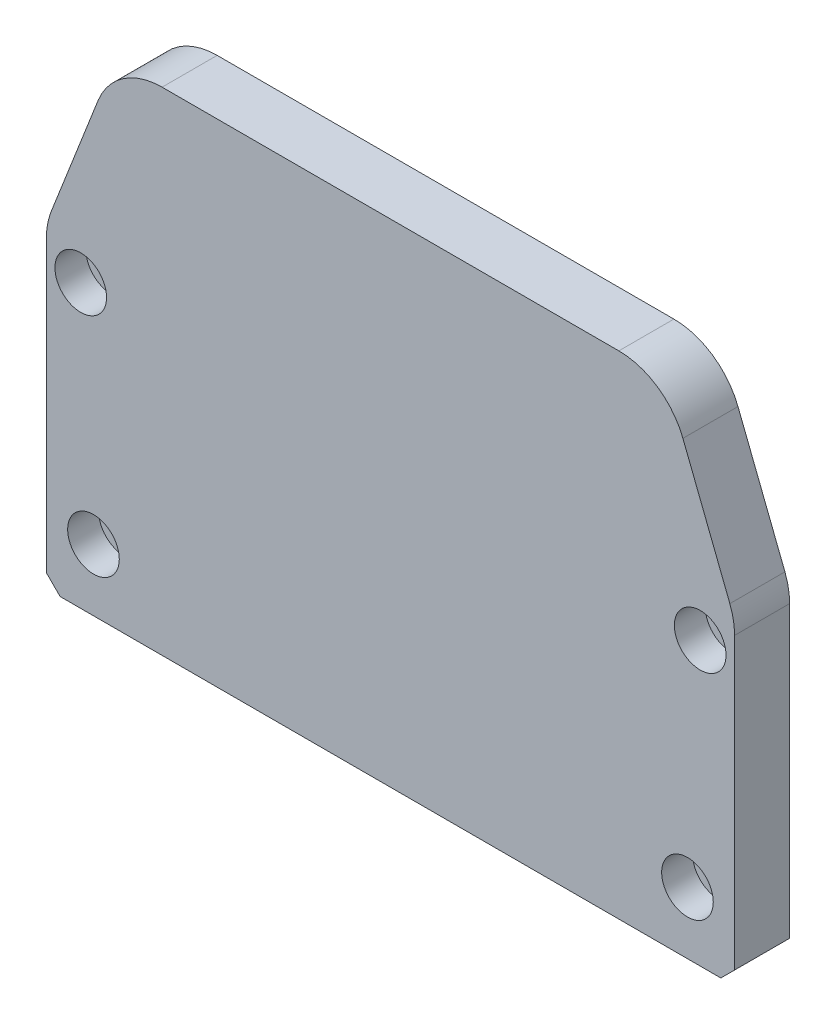
from build123d import *

# Parameters (mm, degrees)
SKETCH_1_W                = 100
SKETCH_1_H                = 71.5
EXTRUDE_1_DEPTH           = 8
CUT_EXTRUDE_1_DEPTH       = 10
FILLET_1_R                = 10
CHAMFER_2_SIZE            = 2
SKETCH_4_R                = 17.5
CUT_EXTRUDE_2_DEPTH       = 5
HOLE_WIZARD_1_D           = 4.5
HOLE_WIZARD_1_CBORE_D     = 7.5
HOLE_WIZARD_1_CBORE_DEPTH = 4.5


with BuildPart() as part:
    # 草图1 → 凸台-拉伸1 (new body)
    with BuildSketch(Plane.XY):
        Rectangle(SKETCH_1_W, SKETCH_1_H)
    extrude(amount=EXTRUDE_1_DEPTH)

    # 草图3 → 切除-拉伸1 (cut)
    with BuildSketch(Plane(origin=(0, 0, 0), x_dir=(-1, 0, 0), z_dir=(0, 0, -1))):
        Polygon((-50, 10.25), (-40, 35.75), (-50, 35.75), align=None)
        Polygon((50, 35.75), (50, 10.25), (40, 35.75), align=None)
    extrude(amount=-CUT_EXTRUDE_1_DEPTH, mode=Mode.SUBTRACT)

    # 圆角1
    fillet_1_edges = [part.edges().sort_by_distance(p)[0] for p in [
        (50, 10.25, 4),
        (40, 35.75, 4),
        (-40, 35.75, 4),
        (-50, 10.25, 4),
    ]]
    fillet(fillet_1_edges, radius=FILLET_1_R)

    # 倒角2
    chamfer_2_edges = [part.edges().sort_by_distance(p)[0] for p in [
        (50, -35.75, 4),
        (-50, -35.75, 4),
    ]]
    chamfer(chamfer_2_edges, length=CHAMFER_2_SIZE)

    # 草图4 → 切除-拉伸2 (cut)
    with BuildSketch(Plane(origin=(0, 0, 0), x_dir=(-1, 0, 0), z_dir=(0, 0, -1))):
        with Locations((0, 8.75)):
            Circle(SKETCH_4_R)
    extrude(amount=-CUT_EXTRUDE_2_DEPTH, mode=Mode.SUBTRACT)

    # 打孔尺寸(%根据)内六角圆柱头螺钉的类型1 (through all)
    with Locations(Plane.XY.offset(8)):
        with Locations((-45, 5.25), (-43.15, -26.75), (45, 5.25), (43.15, -26.75)):
            CounterBoreHole(HOLE_WIZARD_1_D / 2, HOLE_WIZARD_1_CBORE_D / 2, HOLE_WIZARD_1_CBORE_DEPTH)


solid = part.part
